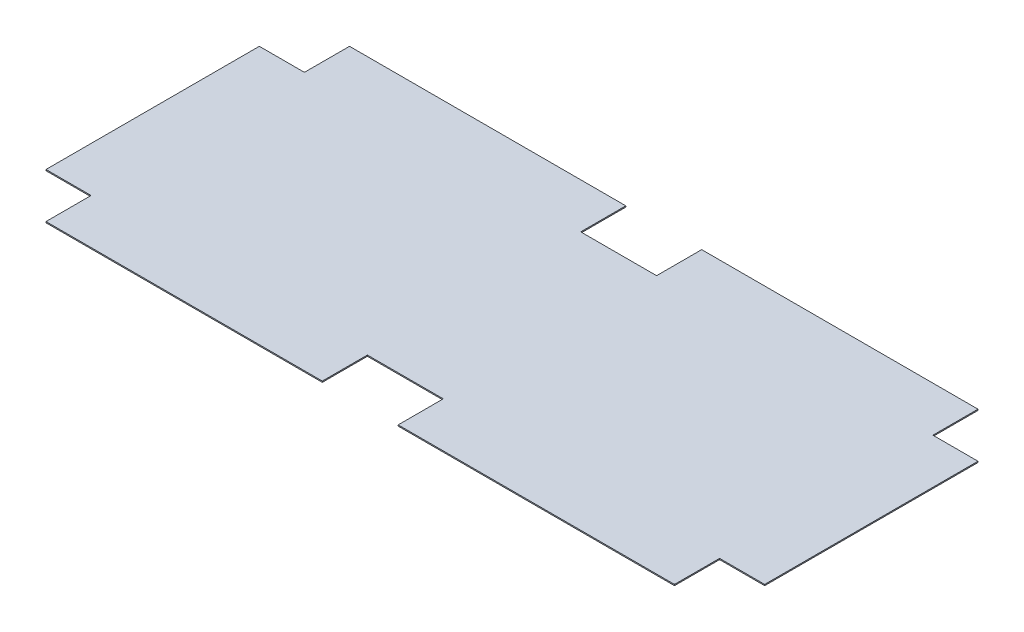
SolidWorks part; units mm, degrees
ref_plane "Front Plane" through (0, 0, 0) normal (0, 0, 1) x (1, 0, 0)
ref_plane "Top Plane" through (0, 0, 0) normal (0, 1, 0) x (1, 0, 0)
ref_plane "Right Plane" through (0, 0, 0) normal (1, 0, 0) x (0, 0, -1)
sketch "Sketch 1" plane through (0, 0, 0) normal (0, 1, 0) x (1, 0, 0)
  line L0 (0, 1610.1852) -> (0, -1740.3704) construction
  line L1 (-3495.168, 0) -> (3807.744, 0) construction
  line L2 (2195, 1060) -> (265, 1060)
  line L3 (-2195, 1060) -> (-2195, 745)
  line L4 (-2195, 745) -> (-2510, 745)
  line L5 (-2510, 745) -> (-2510, -745)
  line L6 (-2195, -745) -> (-2510, -745)
  line L7 (-2195, -1060) -> (-2195, -745)
  line L8 (2195, -1060) -> (265, -1060)
  line L9 (2195, -1060) -> (2195, -745)
  line L10 (2195, -745) -> (2510, -745)
  line L11 (2510, 745) -> (2510, -745)
  line L12 (2195, 745) -> (2510, 745)
  line L13 (2195, 1060) -> (2195, 745)
  line L14 (-265, 1060) -> (-265, 745)
  line L15 (-265, 745) -> (265, 745)
  line L16 (265, 1060) -> (265, 745)
  line L17 (-265, 1060) -> (-2195, 1060)
  line L18 (265, -1060) -> (265, -745)
  line L19 (-265, -745) -> (265, -745)
  line L20 (-265, -1060) -> (-265, -745)
  line L21 (-265, -1060) -> (-2195, -1060)
  point P5 (2510, 0)
  point P13 (-2510, 0)
  point P17 (0, -1060)
  point P22 (0, 1060)
  point P25 (0, 745)
  dimension "D1" = 315
  dimension "D2" = 4390
  dimension "D3" = 5020
  dimension "D4" = 2120
  dimension "D5" = 265
extrude "Boss-Extrude 1" add sketch "Sketch 1" along normal blind 8
